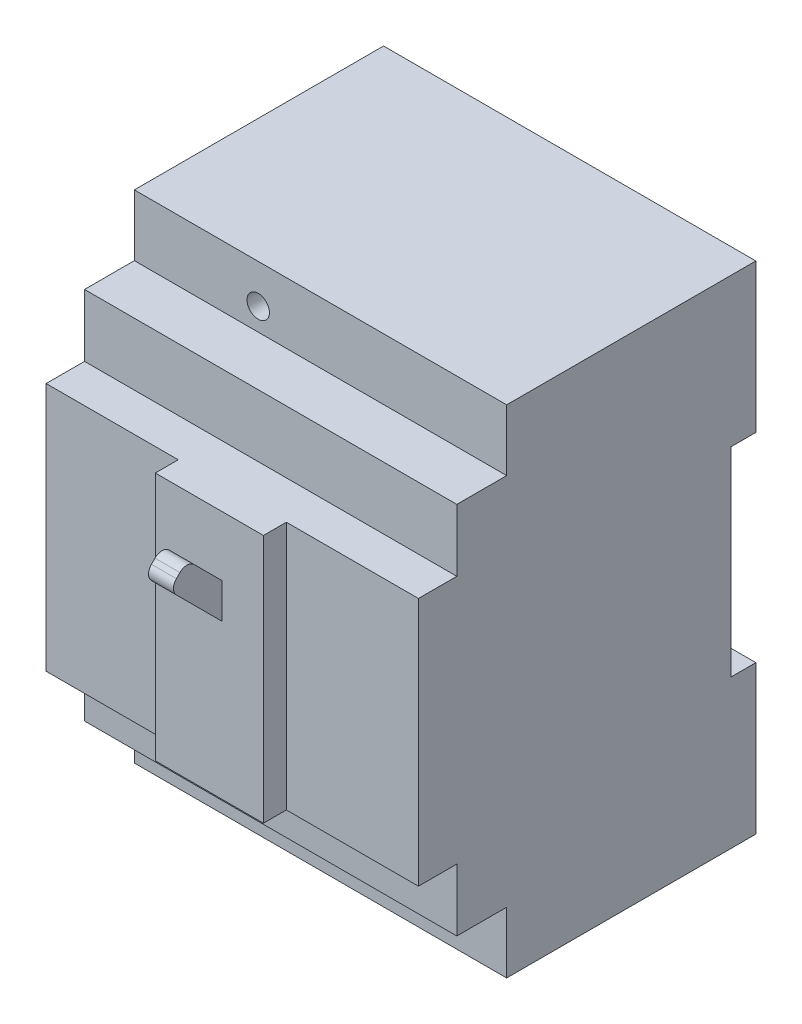
SolidWorks part; units mm, degrees
material "S45C"
ref_plane "Front Plane" through (0, 0, 0) normal (0, 0, 1) x (1, 0, 0)
ref_plane "Top Plane" through (0, 0, 0) normal (0, 1, 0) x (1, 0, 0)
ref_plane "Right Plane" through (0, 0, 0) normal (1, 0, 0) x (0, 0, -1)
sketch "Sketch1" plane through (0, 0, 0) normal (0, 0, 1) x (1, 0, 0)
  line L1 (-37.35, 49.8) -> (37.35, 49.8)
  line L2 (-37.35, 49.8) -> (-37.35, -49.8)
  line L3 (-37.35, -49.8) -> (37.35, -49.8)
  line L4 (37.35, 49.8) -> (37.35, -49.8)
  line L5 (-37.35, 49.8) -> (37.35, -49.8) construction
  line L6 (-37.35, -49.8) -> (37.35, 49.8) construction
  point P0 (0, 0)
  dimension "D1" = 74.7
  dimension "D2" = 99.6
extrude "Boss-Extrude1" add sketch "Sketch1" along normal mid plane 67.7
hole_wizard "Ø4.5 (4.5) Diameter Hole1" positions "Sketch3" profile "Sketch2" hole size "Ø4.5" standard "GB" end condition through all
sketch "Sketch3" plane through (0, 0, 33.85) normal (0, 0, 1) x (1, 0, 0)
  line L0 (0, 0) -> (0, 60.4109) construction
  line L1 (0, 0) -> (-44.7165, 0) construction
  point P0 (-12.5, 42)
  point P3 (12.5, -42)
  dimension "D1" = 84
  dimension "D2" = 42
  dimension "D3" = 25
  dimension "D4" = 12.5
sketch "Sketch2" plane through (-12.5, 42, 33.85) normal (1, 0, 0) x (0, -1, 0)
  line L0 (0, 0) -> (0, 67.7)
  line L1 (0, 67.7) -> (2.25, 67.7)
  line L2 (2.25, 67.7) -> (2.25, 0)
  line L5 (2.25, 0) -> (0, 0)
  line L11 (0, -6.35) -> (0, 107.95) construction
  dimension "通孔孔直径" = 4.5
  dimension "通孔孔深度" = 67.7
sketch "Sketch4" plane through (0, 0, 33.85) normal (0, 0, 1) x (1, 0, 0)
  line L0 (37.35, -49.8) -> (37.35, 49.8) construction
  line L1 (-37.35, 49.8) -> (37.35, 49.8)
  line L2 (-37.35, 49.8) -> (-37.35, 37.5)
  line L3 (-37.35, 37.5) -> (37.35, 37.5)
  line L4 (37.35, 49.8) -> (37.35, 37.5)
  line L5 (0, 0) -> (29.8379, 0) construction
  line L6 (37.35, -49.8) -> (37.35, -37.5)
  line L7 (-37.35, -37.5) -> (37.35, -37.5)
  line L8 (-37.35, -49.8) -> (-37.35, -37.5)
  line L9 (-37.35, -49.8) -> (37.35, -49.8)
  dimension "D1" = 75
extrude "Cut-Extrude1" cut sketch "Sketch4" against normal blind 17.7
sketch "Sketch5" plane through (0, 0, 33.85) normal (0, 0, 1) x (1, 0, 0)
  line L0 (37.35, -37.5) -> (37.35, 37.5) construction
  line L1 (-37.35, -37.5) -> (37.35, -37.5)
  line L2 (-37.35, -37.5) -> (-37.35, -25)
  line L3 (-37.35, -25) -> (37.35, -25)
  line L4 (37.35, -37.5) -> (37.35, -25)
  line L5 (0, 0) -> (-35.3467, 0) construction
  line L6 (37.35, 37.5) -> (37.35, 25)
  line L7 (-37.35, 25) -> (37.35, 25)
  line L8 (-37.35, 37.5) -> (-37.35, 25)
  line L9 (-37.35, 37.5) -> (37.35, 37.5)
  dimension "D1" = 50
extrude "Cut-Extrude2" cut sketch "Sketch5" against normal blind 7.7
sketch "Sketch6" plane through (0, 0, 33.85) normal (0, 0, 1) x (1, 0, 0)
  line L0 (-37.35, 25) -> (37.35, 25) construction
  line L1 (-10.85, -25) -> (10.85, -25)
  line L2 (-10.85, -25) -> (-10.85, 25)
  line L3 (-10.85, 25) -> (10.85, 25)
  line L4 (10.85, -25) -> (10.85, 25)
  line L5 (-10.85, -25) -> (10.85, 25) construction
  line L6 (-10.85, 25) -> (10.85, -25) construction
  point P0 (0, 0)
  dimension "D1" = 21.7
extrude "Boss-Extrude2" add sketch "Sketch6" along normal blind 4.6
sketch "Sketch7" plane through (37.35, 0, 0) normal (1, 0, 0) x (0, 0, -1)
  line L0 (33.85, -49.8) -> (33.85, 49.8) construction
  line L1 (33.85, -20) -> (28.85, -20)
  line L2 (33.85, -20) -> (33.85, 20)
  line L3 (33.85, 20) -> (28.85, 20)
  line L4 (28.85, -20) -> (28.85, 20)
  dimension "D1" = 5
  dimension "D2" = 40
  dimension "D3" = 20
extrude "Cut-Extrude3" cut sketch "Sketch7" against normal blind 118.6
sketch "Sketch8" plane through (0, 0, 0) normal (1, 0, 0) x (0, 0, -1)
  line L0 (-38.45, 13) -> (-45.45, 20)
  line L1 (-38.45, 25) -> (-38.45, -25) construction
  line L2 (-45.45, 20) -> (-48.9855, 16.4645)
  line L3 (-48.9855, 16.4645) -> (-38.45, 5.9289)
  line L4 (-38.45, 13) -> (-38.45, 5.9289)
  line L5 (-38.45, 25) -> (-33.85, 25) construction
  dimension "D1" = 45
  dimension "D2" = 7
  dimension "D3" = 12
  dimension "D4" = 5
extrude "Boss-Extrude3" add sketch "Sketch8" along normal mid plane 5
fillet "Fillet1" radius 2 2 edges at (0, 16.4645, 48.9855) (0, 20, 45.45)
